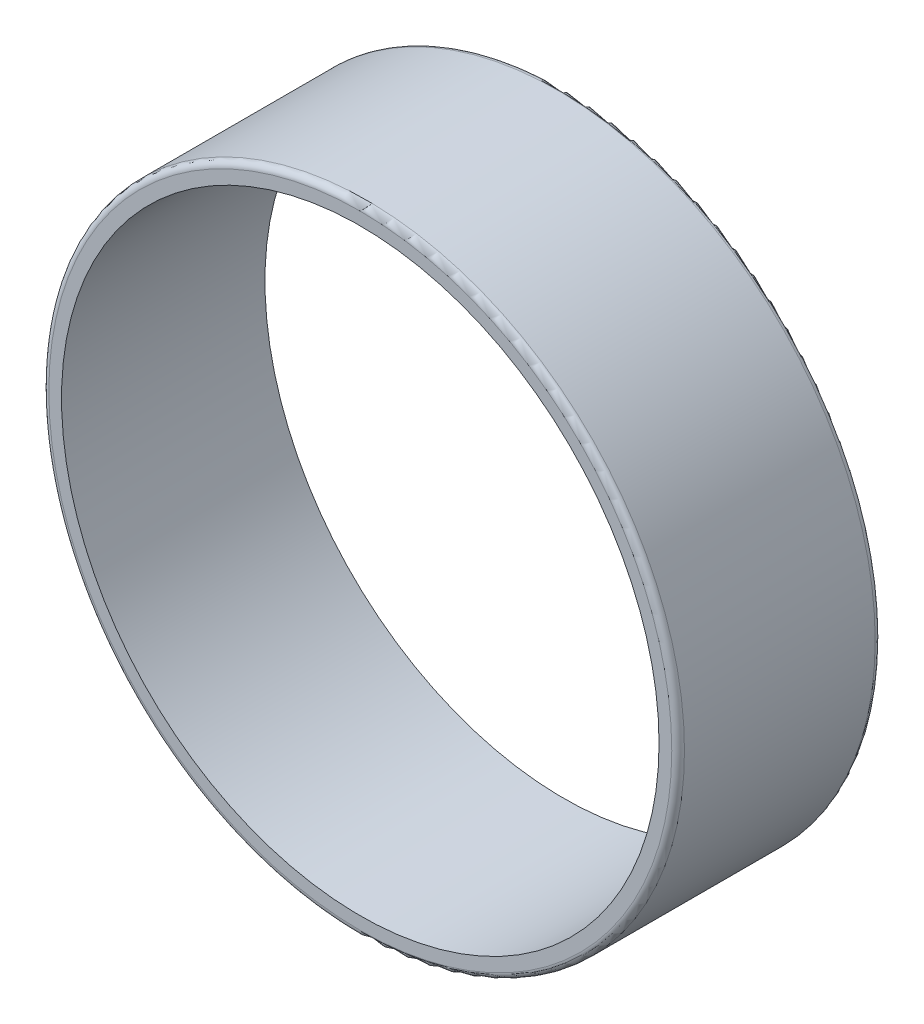
SolidWorks part; units mm, degrees
ref_plane "Front Plane" through (0, 0, 0) normal (0, 0, 1) x (1, 0, 0)
ref_plane "Top Plane" through (0, 0, 0) normal (0, 1, 0) x (1, 0, 0)
ref_plane "Right Plane" through (0, 0, 0) normal (1, 0, 0) x (0, 0, -1)
sketch "Sketch1" plane through (0, 0, 0) normal (0, 0, 1) x (1, 0, 0)
  circle A0 centre (0, 0) radius 47
  circle A1 centre (0, 0) radius 50
  dimension "D1" = 100
  dimension "D2" = 94
extrude "Boss-Extrude1" add sketch "Sketch1" along normal blind 32
fillet "Fillet1" radius 1 2 edges at (50, 0, 0) (50, 0, 32)
